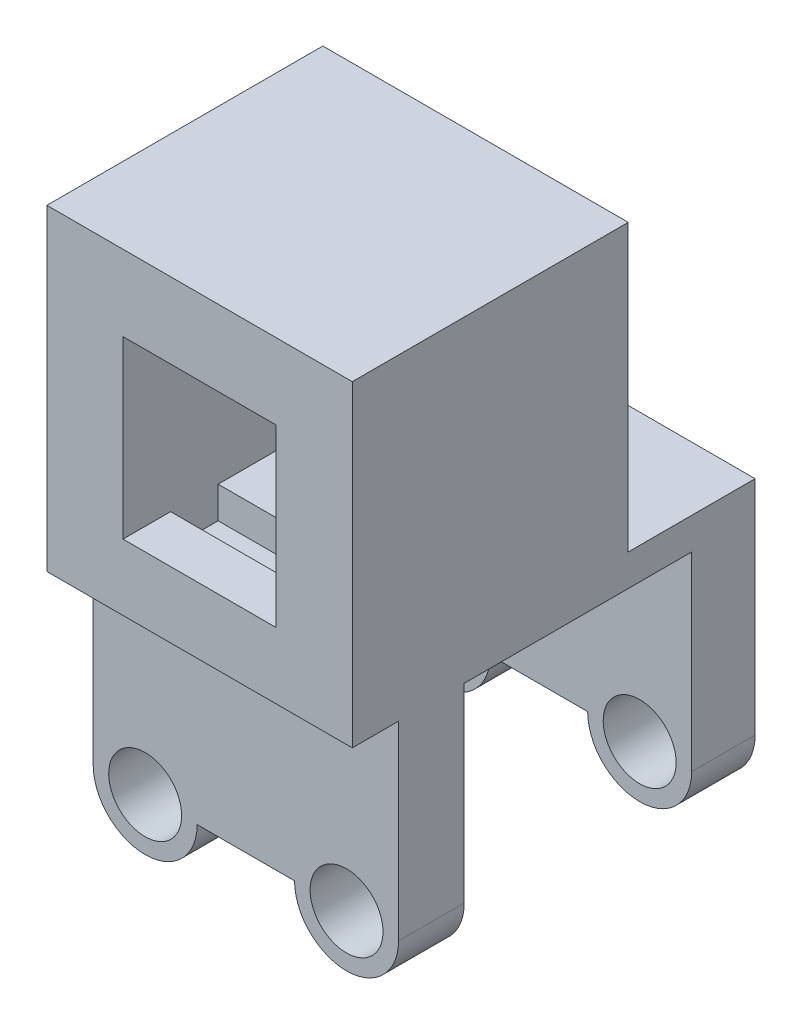
SolidWorks part; units mm, degrees
ref_plane "前视基准面" through (0, 0, 0) normal (0, 0, 1) x (1, 0, 0)
ref_plane "上视基准面" through (0, 0, 0) normal (0, 1, 0) x (1, 0, 0)
ref_plane "右视基准面" through (0, 0, 0) normal (1, 0, 0) x (0, 0, -1)
sketch "草图1" plane through (0, 0, 0) normal (0, 0, 1) x (1, 0, 0)
  line L0 (-3.175, 9.3734) -> (-3.175, -4.8158) construction
  circle A0 centre (0, 0) radius 1.15
  circle A1 centre (0, 0) radius 1.64
  circle A2 centre (-6.35, 0) radius 1.64
  circle A3 centre (-6.35, 0) radius 1.15
  dimension "D1" = 2.3
  dimension "D2" = 3.28
  dimension "D3" = 3.175
extrude "凸台-拉伸1" add sketch "草图1" along normal blind 3.1
sketch "草图2" plane through (0, 0, 3.1) normal (0, 0, 1) x (1, 0, 0)
  line L0 (-7.99, 0) -> (-7.99, 16)
  line L1 (-4.71, 0) -> (-1.64, 0)
  line L3 (1.64, 16) -> (-7.99, 16)
  line L4 (1.64, 0) -> (1.64, 16)
  circle A2 centre (-6.35, 0) radius 1.64 construction
  arc A3 (-4.71, 0) -> (-7.99, 0) centre (-6.35, 0) ccw
  arc A4 (1.64, 0) -> (-1.64, 0) centre (0, 0) ccw
  dimension "D1" = 16
extrude "凸台-拉伸2" add sketch "草图2" against normal up to surface (3.1 mm away) up to face at (-7.99, 0, 0)
sketch "草图4" plane through (0, 0, 3.1) normal (0, 0, 1) x (1, 0, 0)
  line L0 (1.64, 0) -> (1.64, 16) construction
  line L1 (-7.99, 16) -> (1.64, 16)
  line L2 (-7.99, 16) -> (-7.99, 6)
  line L3 (-7.99, 6) -> (1.64, 6)
  line L4 (1.64, 16) -> (1.64, 6)
  dimension "D1" = 10
extrude "凸台-拉伸3" add sketch "草图4" along normal blind 5.6
sketch "草图5" plane through (0, 0, 8.7) normal (0, 0, 1) x (1, 0, 0)
  line L1 (-5.59, 13.615) -> (-0.76, 13.615)
  line L2 (-5.59, 13.615) -> (-5.59, 8.085)
  line L3 (-5.59, 8.085) -> (-0.76, 8.085)
  line L4 (-0.76, 13.615) -> (-0.76, 8.085)
  line L6 (-7.99, 6) -> (1.64, 6) construction
  dimension "D1" = 5.53
  dimension "D4" = 2.085
extrude "切除-拉伸1" cut sketch "草图5" against normal blind 10
ref_plane "基准面1" through (0, 0, 7.2) normal (0, 0, 1) x (1, 0, 0)
sketch "草图6" plane through (0, 0, 7.2) normal (0, 0, 1) x (1, 0, 0)
  line L12 (-5.59, 7.085) -> (-5.59, 14.615)
  line L15 (-5.59, 14.615) -> (-0.76, 14.615)
  line L16 (-0.76, 14.615) -> (-0.76, 7.085)
  line L17 (-0.76, 7.085) -> (-5.59, 7.085)
extrude "切除-拉伸2" cut sketch "草图6" against normal blind 1.5
sketch "草图7" plane through (-7.99, 0, 0) normal (-1, 0, 0) x (0, 0, 1)
  line L0 (5.1709, -1.64) -> (7.2419, -1.64)
  line L1 (5.1709, -1.64) -> (5.1709, 6)
  line L2 (8.7, 6) -> (3.1, 6) construction
  line L3 (5.1709, 6) -> (7.2419, 6)
  line L4 (7.2419, 6) -> (7.2419, -1.64)
  line L5 (0, 6) -> (-2, 6)
  line L6 (0, 16) -> (0, 0) construction
  line L7 (-4, 6) -> (-4, -1.64)
  line L8 (-4, -1.64) -> (-2, -1.64)
  line L9 (-2, 6) -> (-2, -1.64)
  line L10 (-4, 6) -> (-4, 7)
  line L11 (-4, 7) -> (0, 7)
  line L12 (0, 7) -> (0, 6)
  dimension "D1" = 4
  dimension "D2" = 1
extrude "凸台-拉伸4" add sketch "草图7" against normal up to surface (9.63 mm away) up to face at (1.64, 7.3333, 3.9333)
sketch "草图10" plane through (0, 0, -4) normal (0, 0, -1) x (-1, 0, 0)
  line L0 (7.99, 7) -> (7.99, -1.64) construction
  line L1 (-1.64, -1.64) -> (7.99, -1.64) construction
  circle A0 centre (0, 0) radius 1.15
  circle A4 centre (6.35, 0) radius 1.15
  dimension "D1" = 1.64
  dimension "D3" = 2.3
  dimension "D4" = 2.3
  dimension "D2" = 1.64
extrude "切除-拉伸3" cut sketch "草图10" against normal through all
sketch "草图11" plane through (1.64, 0, 0) normal (1, 0, 0) x (0, 0, -1)
  line L1 (-3.1, 6) -> (0, 6)
  line L2 (-3.1, 6) -> (-3.1, -1.64)
  line L3 (-3.1, -1.64) -> (0, -1.64)
  line L4 (0, 6) -> (0, -1.64)
extrude "切除-拉伸4" cut sketch "草图11" against normal through all
sketch "草图12" plane through (0, 0, -4) normal (0, 0, -1) x (-1, 0, 0)
  line L0 (1.64, 0) -> (4.71, 0)
  line L1 (-1.64, 0) -> (-1.64, -1.64)
  line L2 (-1.64, -1.64) -> (0, -1.64)
  line L3 (0, -1.64) -> (6.35, -1.64)
  line L4 (6.35, -1.64) -> (7.99, -1.64)
  line L5 (7.99, -1.64) -> (7.99, 0)
  arc A0 (-1.64, 0) -> (1.64, 0) centre (0, 0) ccw
  arc A1 (4.71, 0) -> (7.99, 0) centre (6.35, 0) ccw
  line M4 (-1.64, 7) -> (-1.64, -1.64)
  line M5 (-1.64, -1.64) -> (7.99, -1.64)
  line M6 (7.99, -1.64) -> (7.99, 7)
extrude "切除-拉伸5" cut sketch "草图12" against normal through all contours A1 L0 A0 M5 | A0 M4 M5 | A1 M5 M6
